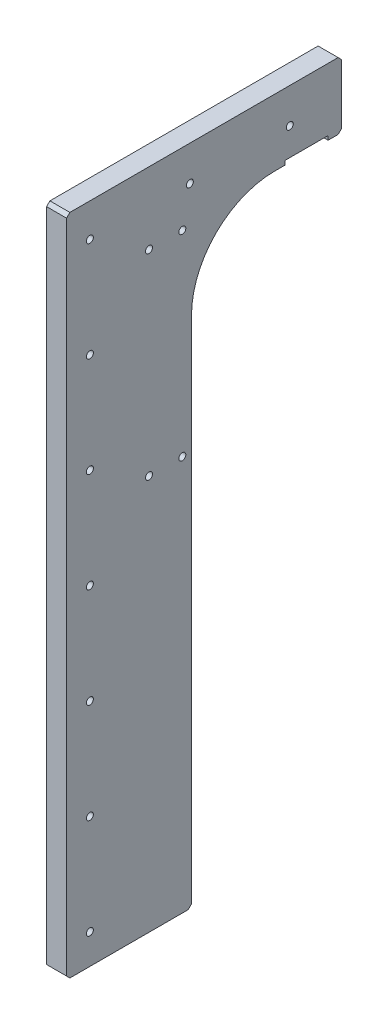
from build123d import *

# Parameters (mm, degrees)
SKETCH1_W              = 75
SKETCH1_H              = 203
BOSS_EXTRUDE1_DEPTH    = 12
SKETCH2_W              = 43
SKETCH2_H              = 70
CUT_EXTRUDE1_DEPTH     = 2
SKETCH3_W              = 12
SKETCH3_H              = 10
BOSS_EXTRUDE2_DEPTH    = 75
SKETCH4_W              = 50
SKETCH4_H              = 60
CUT_EXTRUDE2_DEPTH     = 152.995065709
SKETCH9_R              = 1.5
CUT_EXTRUDE3_DEPTH     = 2
BOSS_EXTRUDE3_DEPTH    = 12
BOSS_EXTRUDE4_DEPTH    = 12
FILLET2_R              = 50
M5_TAPPED_HOLE2_D      = 4.2
LPATTERN4_COUNT        = 7
LPATTERN4_PITCH        = 60
M5_TAPPED_HOLE3_D      = 4.2
LPATTERN5_COUNT        = 2
LPATTERN5_PITCH        = 60
CHAMFER2_SIZE          = 2
CUT_EXTRUDE5_DEPTH     = 1.5
LPATTERN6_COUNT        = 7
LPATTERN6_PITCH        = 60
CUT_EXTRUDE6_DEPTH     = 1.5
SKETCH24_W             = 26
SKETCH24_H             = 10
CUT_EXTRUDE7_DEPTH     = 5
LPATTERN7_COUNT        = 5
LPATTERN7_PITCH        = 60
BOSS_EXTRUDE5_START    = 2
BOSS_EXTRUDE5_DEPTH    = 2
M5_TAPPED_HOLE4_D      = 4.2
M5_TAPPED_HOLE4_DEPTH  = 12.4
M5_TAPPED_HOLE4_TIP    = 1.2618073
FILLET3_R              = 2
LPATTERN8_COUNT        = 6
LPATTERN8_PITCH        = 60
FILLET3_OF_LPATTERN8_R = 2
SKETCH26_W             = 26
SKETCH26_H             = 10
CUT_EXTRUDE8_DEPTH     = 5
SKETCH27_W             = 26
SKETCH27_H             = 2.45
CUT_EXTRUDE9_DEPTH     = 15
FILLET4_R              = 2


with BuildPart() as part:
    # Sketch1 → Boss-Extrude1 (new body)
    with BuildSketch(Plane(origin=(0, 0, 0), x_dir=(0, 0, -1), z_dir=(1, 0, 0))):
        Rectangle(SKETCH1_W, SKETCH1_H)
    extrude(amount=BOSS_EXTRUDE1_DEPTH)

    # Sketch2 → Cut-Extrude1 (cut)
    with BuildSketch(Plane(origin=(12, 0, 0), x_dir=(0, 0, -1), z_dir=(1, 0, 0))):
        with Locations((16, 3.5)):
            Rectangle(SKETCH2_W, SKETCH2_H)
    extrude(amount=-CUT_EXTRUDE1_DEPTH, mode=Mode.SUBTRACT)

    # Sketch3 → Boss-Extrude2 (add)
    with BuildSketch(Plane(origin=(0, 0, -37.5), x_dir=(-1, 0, 0), z_dir=(0, 0, -1))):
        with Locations((-6, 96.5)):
            Rectangle(SKETCH3_W, SKETCH3_H)
    extrude(amount=BOSS_EXTRUDE2_DEPTH)

    # Sketch4 → Cut-Extrude2 (cut, through all)
    with BuildSketch(Plane(origin=(12, 0, 0), x_dir=(0, 0, -1), z_dir=(1, 0, 0))):
        with Locations((12.5, -71.5)):
            Rectangle(SKETCH4_W, SKETCH4_H)
    extrude(amount=-CUT_EXTRUDE2_DEPTH, mode=Mode.SUBTRACT)

    # Sketch9 → Cut-Extrude3 (cut)
    with BuildSketch(Plane(origin=(12, 0, 0), x_dir=(0, 0, -1), z_dir=(1, 0, 0))):
        with Locations((-5.5, 38.5)):
            Circle(SKETCH9_R)
        with Locations((-5.5, -31.5)):
            Circle(SKETCH9_R)
    extrude(amount=-CUT_EXTRUDE3_DEPTH, mode=Mode.SUBTRACT)

    # Sketch10 → Boss-Extrude3 (add)
    with BuildSketch(Plane(origin=(12, 0, 0), x_dir=(0, 0, -1), z_dir=(1, 0, 0))):
        Polygon((-37.5, -101.5), (-12.5, -101.5), (-12.5, -41.5), (37.5, -41.5), (37.5, -266.5), (-37.5, -266.5), align=None)
    extrude(amount=-BOSS_EXTRUDE3_DEPTH)

    # Sketch11 → Boss-Extrude4 (add)
    with BuildSketch(Plane(origin=(12, 0, 0), x_dir=(0, 0, -1), z_dir=(1, 0, 0))):
        Polygon((112.5, 101.5), (112.5, 91.5), (127.5, 91.5), (127.5, 131.5), (-37.5, 131.5), (-37.5, 101.5), align=None)
    extrude(amount=-BOSS_EXTRUDE4_DEPTH)

    # Fillet2
    fillet2_edges = [part.edges().sort_by_distance(p)[0] for p in [
        (6, 91.5, -37.5),
    ]]
    fillet(fillet2_edges, radius=FILLET2_R)

    # M5 Tapped Hole2 (through all)
    with Locations(Plane(origin=(12, 0, 0), x_dir=(0, 0, -1), z_dir=(1, 0, 0))):
        with Locations((-23.5, -248.5)):
            m5_tapped_hole2 = Hole(M5_TAPPED_HOLE2_D / 2)

    # LPattern4: M5 Tapped Hole2 ×7
    with Locations(*[(0, i * LPATTERN4_PITCH, 0) for i in range(1, LPATTERN4_COUNT)]):
        add(m5_tapped_hole2, mode=Mode.SUBTRACT)

    # M5 Tapped Hole3 (through all)
    with Locations(Plane(origin=(12, 0, 0), x_dir=(0, 0, -1), z_dir=(1, 0, 0))):
        with Locations((36.491666088, 110.5)):
            m5_tapped_hole3 = Hole(M5_TAPPED_HOLE3_D / 2)

    # LPattern5: M5 Tapped Hole3 ×2
    with Locations(*[(0, 0, -i * LPATTERN5_PITCH) for i in range(1, LPATTERN5_COUNT)]):
        add(m5_tapped_hole3, mode=Mode.SUBTRACT)

    # Chamfer2
    chamfer2_edges = [part.edges().sort_by_distance(p)[0] for p in [
        (6, 91.5, -127.5),
        (6, 131.5, -127.5),
        (6, 131.5, 37.5),
        (6, -266.5, -37.5),
        (6, -266.5, 37.5),
    ]]
    chamfer(chamfer2_edges, length=CHAMFER2_SIZE)

    # Sketch19 → Cut-Extrude5 (cut)
    with BuildSketch(Plane.ZY):
        with BuildLine():
            Line((31.7, -259.7), (31.7, -238.65))
            ThreePointArc((31.7, -238.65), (30.572361108, -235.927638892), (27.85, -234.8))
            Line((27.85, -234.8), (-0.85, -234.8))
            ThreePointArc((-0.85, -234.8), (-3.572361108, -235.927638892), (-4.7, -238.65))
            Line((-4.7, -238.65), (-4.7, -259.7))
            ThreePointArc((-4.7, -259.7), (-3.572361108, -262.422361108), (-0.85, -263.55))
            Line((-0.85, -263.55), (27.85, -263.55))
            ThreePointArc((27.85, -263.55), (30.572361108, -262.422361108), (31.7, -259.7))
        make_face()
        with BuildLine():
            Line((29.9, -259.7), (29.9, -238.65))
            ThreePointArc((29.9, -238.65), (29.299568901, -237.200431099), (27.85, -236.6))
            Line((27.85, -236.6), (-0.85, -236.6))
            ThreePointArc((-0.85, -236.6), (-2.299568901, -237.200431099), (-2.9, -238.65))
            Line((-2.9, -238.65), (-2.9, -259.7))
            ThreePointArc((-2.9, -259.7), (-2.299568901, -261.149568901), (-0.85, -261.75))
            Line((-0.85, -261.75), (27.85, -261.75))
            ThreePointArc((27.85, -261.75), (29.299568901, -261.149568901), (29.9, -259.7))
        make_face(mode=Mode.SUBTRACT)
    cut_extrude5 = extrude(amount=-CUT_EXTRUDE5_DEPTH, mode=Mode.SUBTRACT)

    # LPattern6: Cut-Extrude5 ×7
    with Locations(*[(0, i * LPATTERN6_PITCH, 0) for i in range(1, LPATTERN6_COUNT)]):
        add(cut_extrude5, mode=Mode.SUBTRACT)

    # Sketch20 → Cut-Extrude6 (cut)
    with BuildSketch(Plane.ZY):
        with BuildLine():
            Line((-64.7, 121.35), (-64.7, 100.3))
            ThreePointArc((-64.7, 100.3), (-63.572361108, 97.577638892), (-60.85, 96.45))
            Line((-60.85, 96.45), (-32.15, 96.45))
            ThreePointArc((-32.15, 96.45), (-29.427638892, 97.577638892), (-28.3, 100.3))
            Line((-28.3, 100.3), (-28.3, 121.35))
            ThreePointArc((-28.3, 121.35), (-29.427638892, 124.072361108), (-32.15, 125.2))
            Line((-32.15, 125.2), (-60.85, 125.2))
            ThreePointArc((-60.85, 125.2), (-63.572361108, 124.072361108), (-64.7, 121.35))
        make_face()
        with BuildLine():
            Line((-62.9, 121.35), (-62.9, 100.3))
            ThreePointArc((-62.9, 100.3), (-62.299568901, 98.850431099), (-60.85, 98.25))
            Line((-60.85, 98.25), (-32.15, 98.25))
            ThreePointArc((-32.15, 98.25), (-30.700431099, 98.850431099), (-30.1, 100.3))
            Line((-30.1, 100.3), (-30.1, 121.35))
            ThreePointArc((-30.1, 121.35), (-30.700431099, 122.799568901), (-32.15, 123.4))
            Line((-32.15, 123.4), (-60.85, 123.4))
            ThreePointArc((-60.85, 123.4), (-62.299568901, 122.799568901), (-62.9, 121.35))
        make_face(mode=Mode.SUBTRACT)
    cut_extrude6 = extrude(amount=-CUT_EXTRUDE6_DEPTH, mode=Mode.SUBTRACT)

    # Sketch24 → Cut-Extrude7 (cut)
    with BuildSketch(Plane.ZY):
        with Locations((13.5, -211.05)):
            Rectangle(SKETCH24_W, SKETCH24_H)
    cut_extrude7 = extrude(amount=-CUT_EXTRUDE7_DEPTH, mode=Mode.SUBTRACT)

    # LPattern7: Cut-Extrude6 ×5
    with Locations(*[(0, 0, -i * LPATTERN7_PITCH) for i in range(1, LPATTERN7_COUNT)]):
        add(cut_extrude6, mode=Mode.SUBTRACT)

    # Sketch21 → Boss-Extrude5 (add)
    with BuildSketch(Plane(origin=(10, 0, 0), x_dir=(0, 0, -1), z_dir=(1, 0, 0)).offset(BOSS_EXTRUDE5_START)):
        with BuildLine():
            Line((-4, -31.5), (37.5, -31.5))
            Line((37.5, -31.5), (37.5, 38.5))
            Line((37.5, 38.5), (-4, 38.5))
            ThreePointArc((-4, 38.5), (-6.560660172, 39.560660172), (-5.5, 37))
            Line((-5.5, 37), (-5.5, -30))
            ThreePointArc((-5.5, -30), (-6.560660172, -32.560660172), (-4, -31.5))
        make_face()
    extrude(amount=-BOSS_EXTRUDE5_DEPTH)

    # M5 Tapped Hole4
    with Locations(Plane(origin=(12, 0, 0), x_dir=(0, 0, -1), z_dir=(1, 0, 0))):
        with Locations((12, 88.45), (32, 88.45), (12, -29.25), (32, -29.25)):
            Hole(M5_TAPPED_HOLE4_D / 2, depth=M5_TAPPED_HOLE4_DEPTH)
            with Locations((0, 0, -(M5_TAPPED_HOLE4_DEPTH + M5_TAPPED_HOLE4_TIP / 2))):  # 118° drill point
                Cone(0, M5_TAPPED_HOLE4_D / 2, M5_TAPPED_HOLE4_TIP, mode=Mode.SUBTRACT)

    # Fillet3
    fillet3_edges = [part.edges().sort_by_distance(p)[0] for p in [
        (2.5, -216.05, 0.5),
        (2.5, -206.05, 0.5),
        (2.5, -206.05, 26.5),
        (2.5, -216.05, 26.5),
    ]]
    fillet(fillet3_edges, radius=FILLET3_R)

    # LPattern8: Cut-Extrude7 ×6
    with Locations(*[(0, i * LPATTERN8_PITCH, 0) for i in range(1, LPATTERN8_COUNT)]):
        add(cut_extrude7, mode=Mode.SUBTRACT)

    # Fillet3 of LPattern8
    fillet3_of_lpattern8_edges = [part.edges().sort_by_distance(p)[0] for p in [
        (2.5, -156.05, 0.5),
        (2.5, -146.05, 0.5),
        (2.5, -146.05, 26.5),
        (2.5, -156.05, 26.5),
        (2.5, -96.05, 0.5),
        (2.5, -86.05, 0.5),
        (2.5, -86.05, 26.5),
        (2.5, -96.05, 26.5),
        (2.5, -36.05, 0.5),
        (2.5, -26.05, 0.5),
        (2.5, -26.05, 26.5),
        (2.5, -36.05, 26.5),
        (2.5, 23.95, 0.5),
        (2.5, 33.95, 0.5),
        (2.5, 33.95, 26.5),
        (2.5, 23.95, 26.5),
        (2.5, 83.95, 0.5),
        (2.5, 93.95, 0.5),
        (2.5, 93.95, 26.5),
        (2.5, 83.95, 26.5),
    ]]
    fillet(fillet3_of_lpattern8_edges, radius=FILLET3_OF_LPATTERN8_R)

    # Sketch26 → Cut-Extrude8 (cut)
    with BuildSketch(Plane.ZY):
        with Locations((-46.5, 88.95)):
            Rectangle(SKETCH26_W, SKETCH26_H)
    extrude(amount=-CUT_EXTRUDE8_DEPTH, mode=Mode.SUBTRACT)

    # Sketch27 → Cut-Extrude9 (cut)
    with BuildSketch(Plane.ZY):
        with Locations((-106.5, 92.725)):
            Rectangle(SKETCH27_W, SKETCH27_H)
    extrude(amount=-CUT_EXTRUDE9_DEPTH, mode=Mode.SUBTRACT)

    # Fillet4
    fillet4_edges = [part.edges().sort_by_distance(p)[0] for p in [
        (2.5, 93.95, -33.5),
        (2.5, 83.95, -59.5),
        (2.5, 93.95, -59.5),
        (2.5, 83.95, -33.5),
    ]]
    fillet(fillet4_edges, radius=FILLET4_R)


solid = part.part
